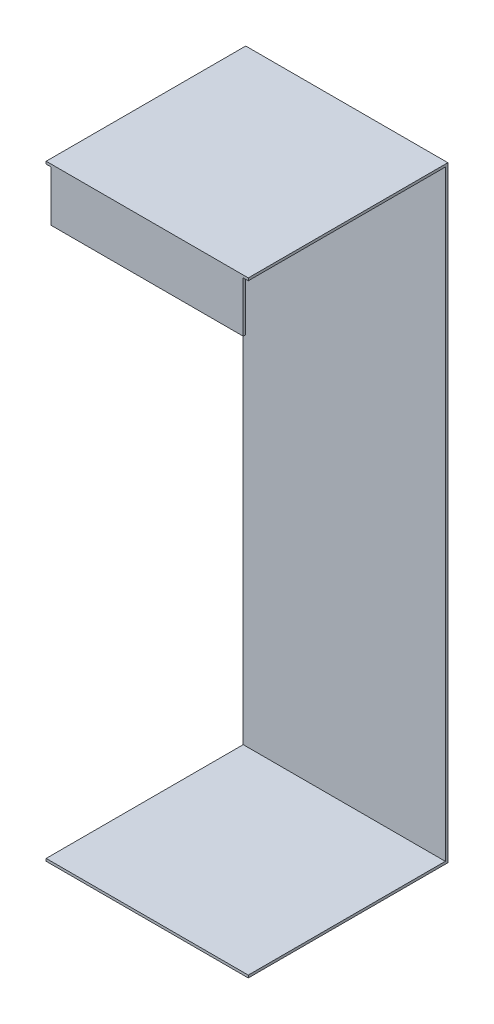
from build123d import *

# Parameters (mm, degrees)
SKETCH1_W           = 80
SKETCH1_H           = 240
BOSS_EXTRUDE1_DEPTH = 1
SKETCH2_W           = 80
SKETCH2_H           = 1
BOSS_EXTRUDE2_DEPTH = 78
SKETCH3_W           = 80
SKETCH3_H           = 20
BOSS_EXTRUDE3_DEPTH = 1
SKETCH4_W           = 2
SKETCH4_H           = 1
CUT_EXTRUDE1_DEPTH  = 20


with BuildPart() as part:
    # Sketch1 → Boss-Extrude1 (new body)
    with BuildSketch(Plane.XY):
        Rectangle(SKETCH1_W, SKETCH1_H)
    extrude(amount=BOSS_EXTRUDE1_DEPTH)

    # Sketch2 → Boss-Extrude2 (add)
    with BuildSketch(Plane.XY.offset(1)):
        with Locations((0, 119.5)):
            Rectangle(SKETCH2_W, SKETCH2_H)
        with Locations((0, -119.5)):
            Rectangle(SKETCH2_W, SKETCH2_H)
    extrude(amount=BOSS_EXTRUDE2_DEPTH)

    # Sketch3 → Boss-Extrude3 (add)
    with BuildSketch(Plane.XY.offset(79)):
        with Locations((0, 109)):
            Rectangle(SKETCH3_W, SKETCH3_H)
    extrude(amount=-BOSS_EXTRUDE3_DEPTH)

    # Sketch4 → Cut-Extrude1 (cut)
    with BuildSketch(Plane(origin=(0, 99, 0), x_dir=(1, 0, 0), z_dir=(0, 1, 0))):
        with Locations((-39, -78.5)):
            Rectangle(SKETCH4_W, SKETCH4_H)
        with Locations((39, -78.5)):
            Rectangle(SKETCH4_W, SKETCH4_H)
    extrude(amount=CUT_EXTRUDE1_DEPTH, mode=Mode.SUBTRACT)


solid = part.part
